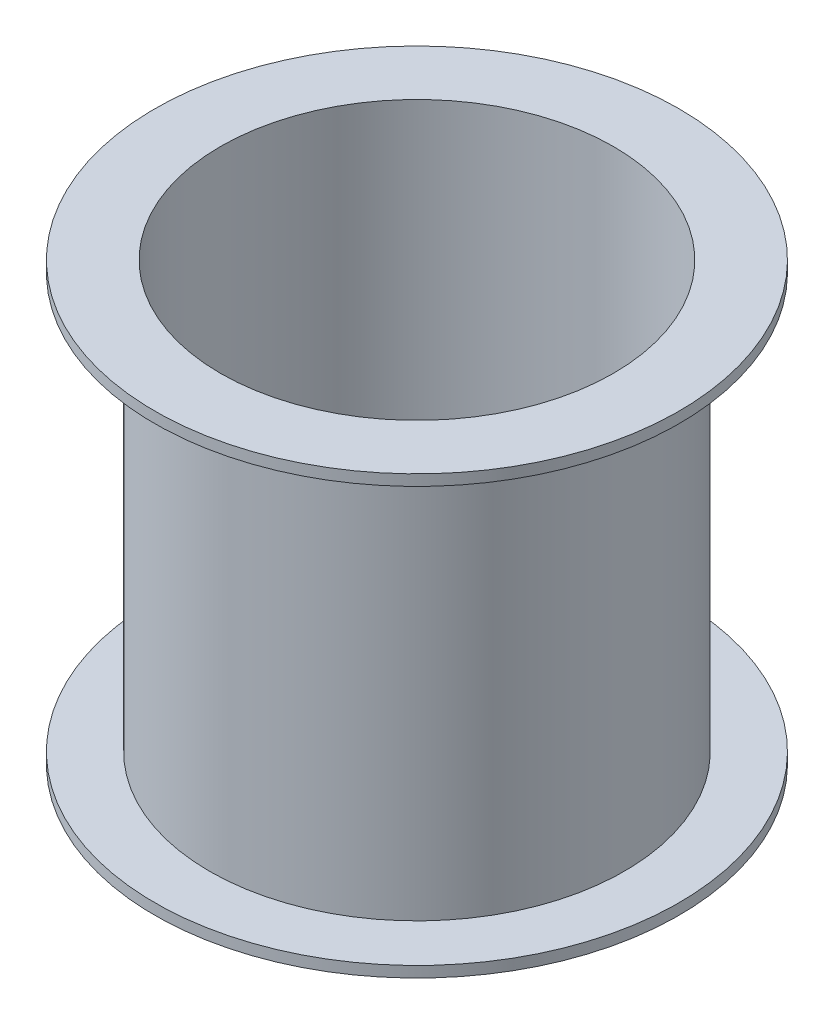
SolidWorks part; units mm, degrees
ref_plane "Front Plane" through (0, 0, 0) normal (0, 0, 1) x (1, 0, 0)
ref_plane "Top Plane" through (0, 0, 0) normal (0, 1, 0) x (1, 0, 0)
ref_plane "Right Plane" through (0, 0, 0) normal (1, 0, 0) x (0, 0, -1)
other "Configuration Table"
sketch "Sketch2" plane through (0, 0, 0) normal (1, 0, 0) x (0, 0, -1)
  line L0 (0, 0) -> (0, 40)
  line L2 (24, 40) -> (24, 39)
  line L3 (24, 39) -> (19, 39)
  line L4 (19, 39) -> (19, 1)
  line L5 (19, 1) -> (24, 1)
  line L6 (24, 1) -> (24, 0)
  line L8 (24, 40) -> (18, 40)
  line L9 (18, 40) -> (18, 0)
  line L10 (18, 0) -> (24, 0)
  dimension "D1" = 24
  dimension "D2" = 40
  dimension "D3" = 5
  dimension "D4" = 6
  dimension "D5" = 1
  dimension "D6" = 1
  dimension "D7" = 6
revolve "Revolve2" add sketch "Sketch2" angle 360 about L0
